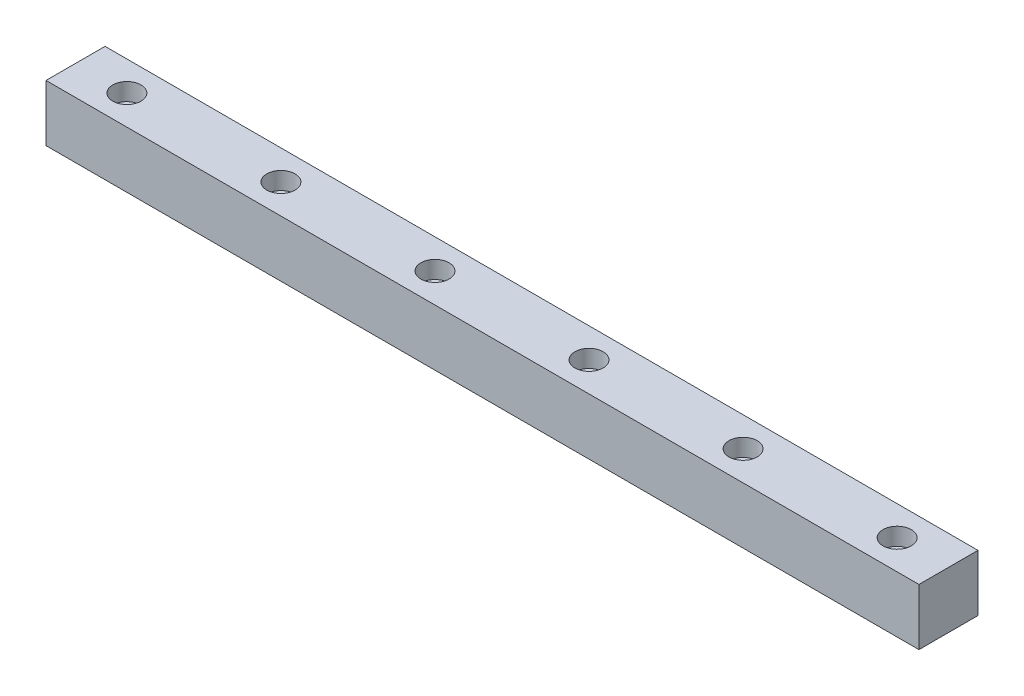
from build123d import *

# Parameters (mm, degrees)
SKETCH_1_W                = 23
SKETCH_1_H                = 22
EXTRUDE_1_DEPTH           = 340
HOLE_WIZARD_1_D           = 6.6
HOLE_WIZARD_1_CBORE_D     = 11
HOLE_WIZARD_1_CBORE_DEPTH = 6.8
PATTERN_LINEAR_2_COUNT    = 6
PATTERN_LINEAR_2_PITCH    = 60


with BuildPart() as part:
    # 草图1 → 凸台-拉伸1 (new body)
    with BuildSketch(Plane(origin=(0, 0, 0), x_dir=(0, 0, -1), z_dir=(1, 0, 0))):
        Rectangle(SKETCH_1_W, SKETCH_1_H)
    extrude(amount=EXTRUDE_1_DEPTH)

    # 打孔尺寸(%根据)内六角圆柱头螺钉的类型1 (through all)
    with Locations(Plane(origin=(0, 11, 0), x_dir=(1, 0, 0), z_dir=(0, 1, 0))):
        with Locations((20, 0)):
            hole_wizard_1 = CounterBoreHole(HOLE_WIZARD_1_D / 2, HOLE_WIZARD_1_CBORE_D / 2, HOLE_WIZARD_1_CBORE_DEPTH)

    # 阵列(线性)2: 打孔尺寸(%根据)内六角圆柱头螺钉的类型1 ×6
    with Locations(*[(i * PATTERN_LINEAR_2_PITCH, 0, 0) for i in range(1, PATTERN_LINEAR_2_COUNT)]):
        add(hole_wizard_1, mode=Mode.SUBTRACT)


solid = part.part
